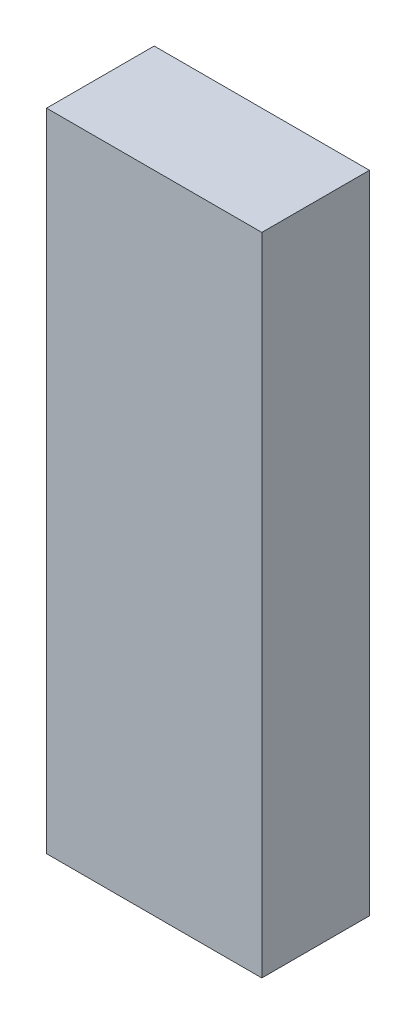
from build123d import *

# Parameters (mm, degrees)
SKETCH_1_W          = 150
SKETCH_1_H          = 60
EXTRUDE_1_DEPTH     = 10
SKETCH_2_W          = 30
SKETCH_2_H          = 80
CUT_EXTRUDE_1_DEPTH = 80
SKETCH_3_W          = 50
SKETCH_3_H          = 60
CUT_EXTRUDE_3_DEPTH = 10


with BuildPart() as part:
    # 草图1 → 凸台-拉伸1 (new body)
    with BuildSketch(Plane.XY):
        with Locations((75, 30)):
            Rectangle(SKETCH_1_W, SKETCH_1_H)
    extrude(amount=EXTRUDE_1_DEPTH)

    # 草图2 → 切除-拉伸1 (cut)
    with BuildSketch(Plane(origin=(150, 0, 0), x_dir=(0, 0, -1), z_dir=(1, 0, 0))):
        with Locations((-5, 30)):
            Rectangle(SKETCH_2_W, SKETCH_2_H)
    extrude(amount=-CUT_EXTRUDE_1_DEPTH, mode=Mode.SUBTRACT)

    # 草图3 → 切除-拉伸3 (cut)
    with BuildSketch(Plane.XY.offset(10)):
        with Locations((45, 30)):
            Rectangle(SKETCH_3_W, SKETCH_3_H)
    extrude(amount=-CUT_EXTRUDE_3_DEPTH, mode=Mode.SUBTRACT)


solid = part.part
